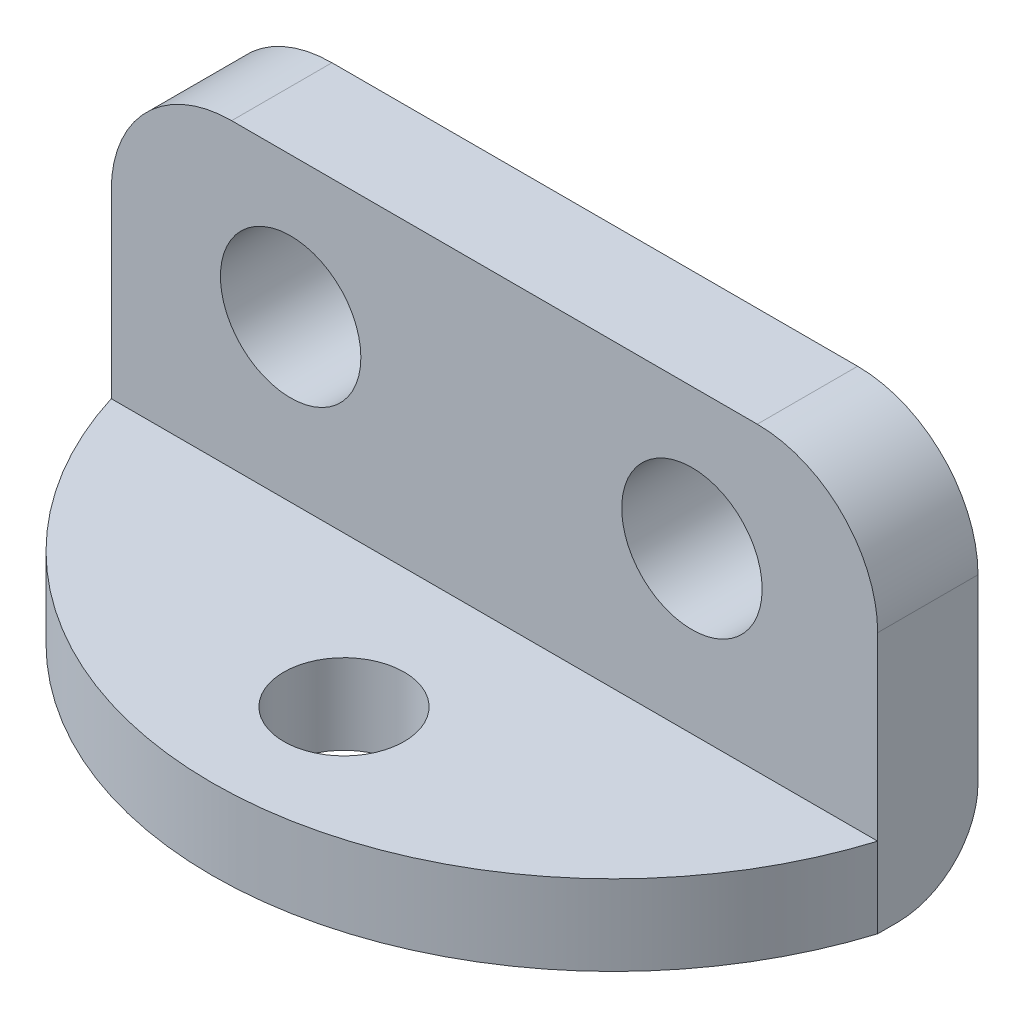
from build123d import *

# Parameters (mm, degrees)
SKETCH_1_R      = 1.75
EXTRUDE_1_DEPTH = 2.5
SKETCH_2_R      = 1.5
EXTRUDE_2_DEPTH = 2
FILLET_1_R      = 2


with BuildPart() as part:
    # 草图1 → 凸台-拉伸1 (new body)
    with BuildSketch(Plane.XY):
        with BuildLine():
            Line((-9.55, -4.75), (9.55, -4.75))
            Line((9.55, -4.75), (9.55, 1.75))
            ThreePointArc((9.55, 1.75), (8.671320344, 3.871320344), (6.55, 4.75))
            Line((6.55, 4.75), (-6.55, 4.75))
            ThreePointArc((-6.55, 4.75), (-8.671320344, 3.871320344), (-9.55, 1.75))
            Line((-9.55, 1.75), (-9.55, -4.75))
        make_face()
        with Locations((4.920618816, 1.25)):
            Circle(SKETCH_1_R, mode=Mode.SUBTRACT)
        with Locations((-5.079381184, 1.25)):
            Circle(SKETCH_1_R, mode=Mode.SUBTRACT)
    extrude(amount=EXTRUDE_1_DEPTH)

    # 草图2 → 凸台-拉伸2 (add)
    with BuildSketch(Plane.XZ.offset(4.75)):
        with BuildLine():
            Line((-9.55, 2.5), (9.55, 2.5))
            ThreePointArc((9.55, 2.5), (0, 9.53394201), (-9.55, 2.5))
        make_face()
        with Locations(Location((0, 6.25, 0), (0, 0, 270))):
            Circle(SKETCH_2_R, mode=Mode.SUBTRACT)
    extrude(amount=-EXTRUDE_2_DEPTH)

    # 圆角1
    fillet_1_edges = [part.edges().sort_by_distance(p)[0] for p in [
        (0, -4.75, 0),
    ]]
    fillet(fillet_1_edges, radius=FILLET_1_R)


solid = part.part
